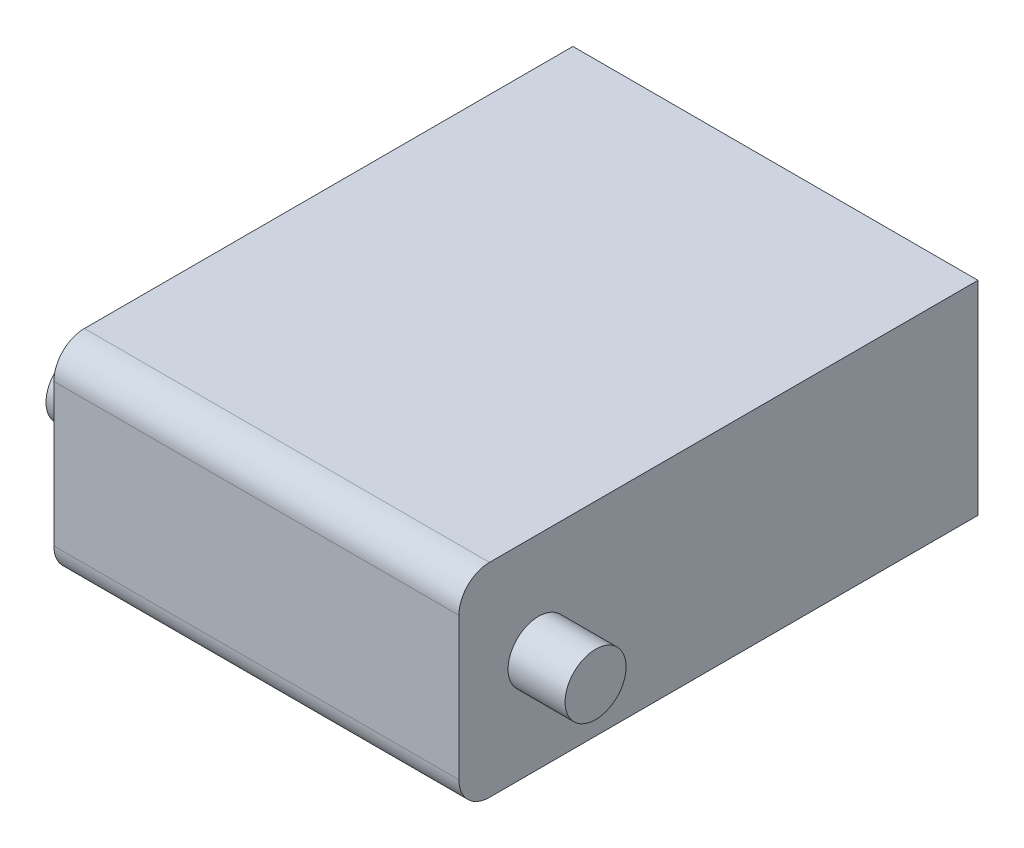
from build123d import *

# Parameters (mm, degrees)
SKETCH1_W             = 39.8
SKETCH1_H             = 20
BOSS_EXTRUDE1_DEPTH   = 51
SKETCH2_R             = 3
BOSS_EXTRUDE2_DEPTH   = 25.5
M3_TAPPED_HOLE1_D     = 2.5
M3_TAPPED_HOLE1_DEPTH = 7.5
M3_TAPPED_HOLE1_TIP   = 0.751075774
FILLET1_R             = 3


with BuildPart() as part:
    # Sketch1 → Boss-Extrude1 (new body)
    with BuildSketch(Plane.XY):
        Rectangle(SKETCH1_W, SKETCH1_H)
    extrude(amount=BOSS_EXTRUDE1_DEPTH)

    # Sketch2 → Boss-Extrude2 (add, symmetric)
    with BuildSketch(Plane(origin=(0, 0, 0), x_dir=(0, 0, -1), z_dir=(1, 0, 0))):
        with Locations(Location((-43.173636791, 0, 0), (0, 0, 90))):
            Circle(SKETCH2_R)
    extrude(amount=BOSS_EXTRUDE2_DEPTH, both=True)

    # M3 Tapped Hole1
    with Locations(Plane(origin=(12.5, 0, 0), x_dir=(-1, 0, 0), z_dir=(0, 0, -1))):
        with Locations((0, 0), (25, 0), (12.62087232, 0)):
            Hole(M3_TAPPED_HOLE1_D / 2, depth=M3_TAPPED_HOLE1_DEPTH)
            with Locations((0, 0, -(M3_TAPPED_HOLE1_DEPTH + M3_TAPPED_HOLE1_TIP / 2))):  # 118° drill point
                Cone(0, M3_TAPPED_HOLE1_D / 2, M3_TAPPED_HOLE1_TIP, mode=Mode.SUBTRACT)

    # Fillet1
    fillet1_edges = [part.edges().sort_by_distance(p)[0] for p in [
        (0, -10, 51),
        (0, 10, 51),
    ]]
    fillet(fillet1_edges, radius=FILLET1_R)


solid = part.part
